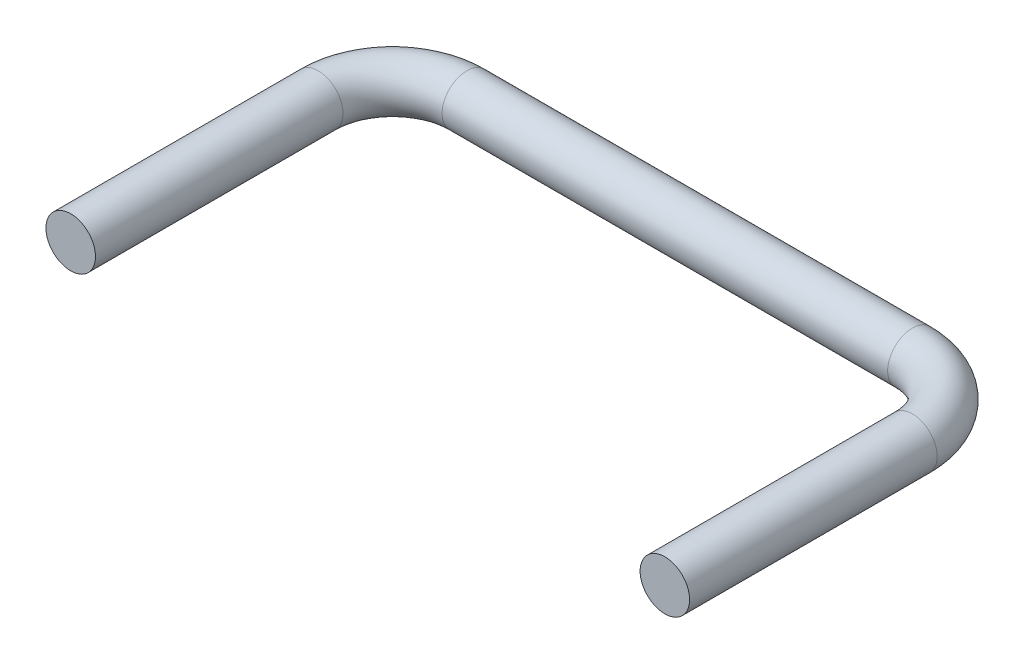
SolidWorks part; units mm, degrees
ref_plane "Front Plane" through (0, 0, 0) normal (0, 0, 1) x (1, 0, 0)
ref_plane "Top Plane" through (0, 0, 0) normal (0, 1, 0) x (1, 0, 0)
ref_plane "Right Plane" through (0, 0, 0) normal (1, 0, 0) x (0, 0, -1)
sketch "Sketch1" plane through (0, 0, 0) normal (0, 0, 1) x (1, 0, 0)
  circle A0 centre (0, 0) radius 6.35
  dimension "D1" = 12.7
sketch "Sketch2" plane through (0, 0, 0) normal (0, 1, 0) x (1, 0, 0)
  line L0 (0, 0) -> (0, 63.5)
  line L1 (19.05, 82.55) -> (133.35, 82.55)
  line L2 (152.4, 63.5) -> (152.4, 0)
  arc A0 (152.4, 63.5) -> (133.35, 82.55) centre (133.35, 63.5) ccw
  arc A1 (19.05, 82.55) -> (0, 63.5) centre (19.05, 63.5) ccw
  point P7 (152.4, 82.55)
  point P10 (0, 82.55)
  dimension "D3" = 19.05
  dimension "D1" = 152.4
  dimension "D2" = 82.55
sweep "Sweep1" add profiles "Sketch1" path "Sketch2"
